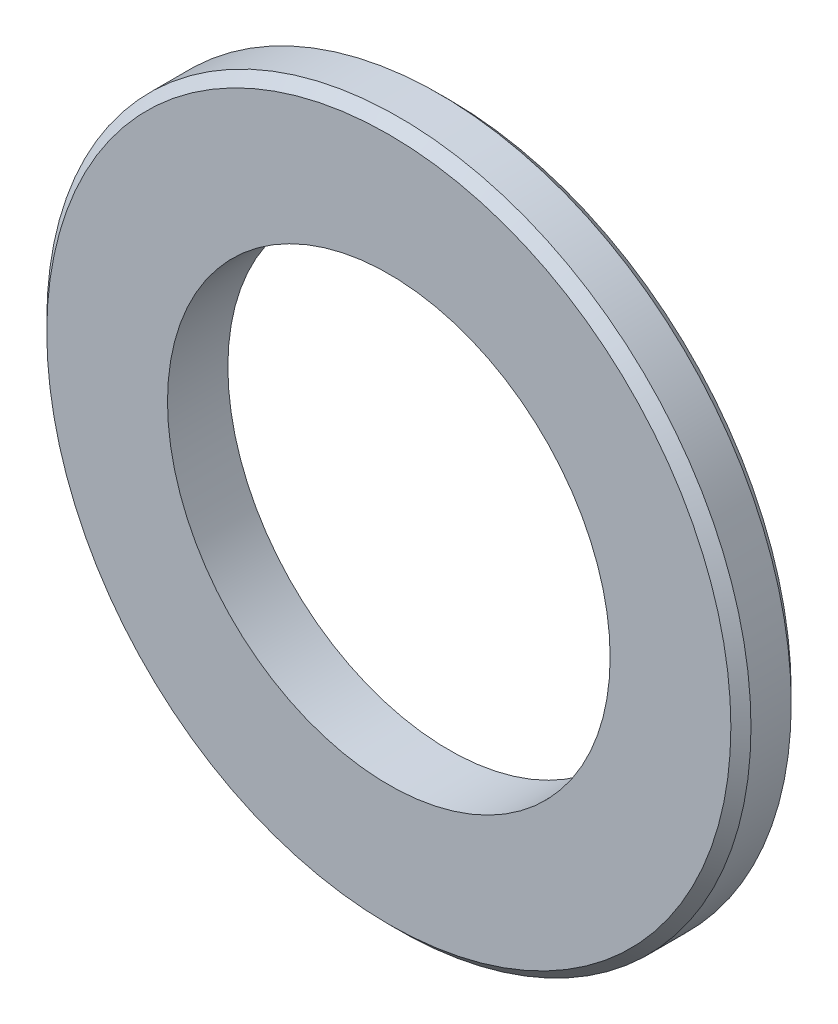
from build123d import *

# Parameters (mm, degrees)
SKETCH_1_R      = 17.5
SKETCH_1_R_2    = 11
EXTRUDE_1_DEPTH = 3
CHAMFER_1_SIZE  = 0.5


with BuildPart() as part:
    # 草图1 → 拉伸1 (new body)
    with BuildSketch(Plane.XY):
        Circle(SKETCH_1_R)
        Circle(SKETCH_1_R_2, mode=Mode.SUBTRACT)
    extrude(amount=EXTRUDE_1_DEPTH)

    # 倒角1
    chamfer_1_edges = [part.edges().sort_by_distance(p)[0] for p in [
        (-17.5, 0, 0),
        (-17.5, 0, 3),
    ]]
    chamfer(chamfer_1_edges, length=CHAMFER_1_SIZE)


solid = part.part
